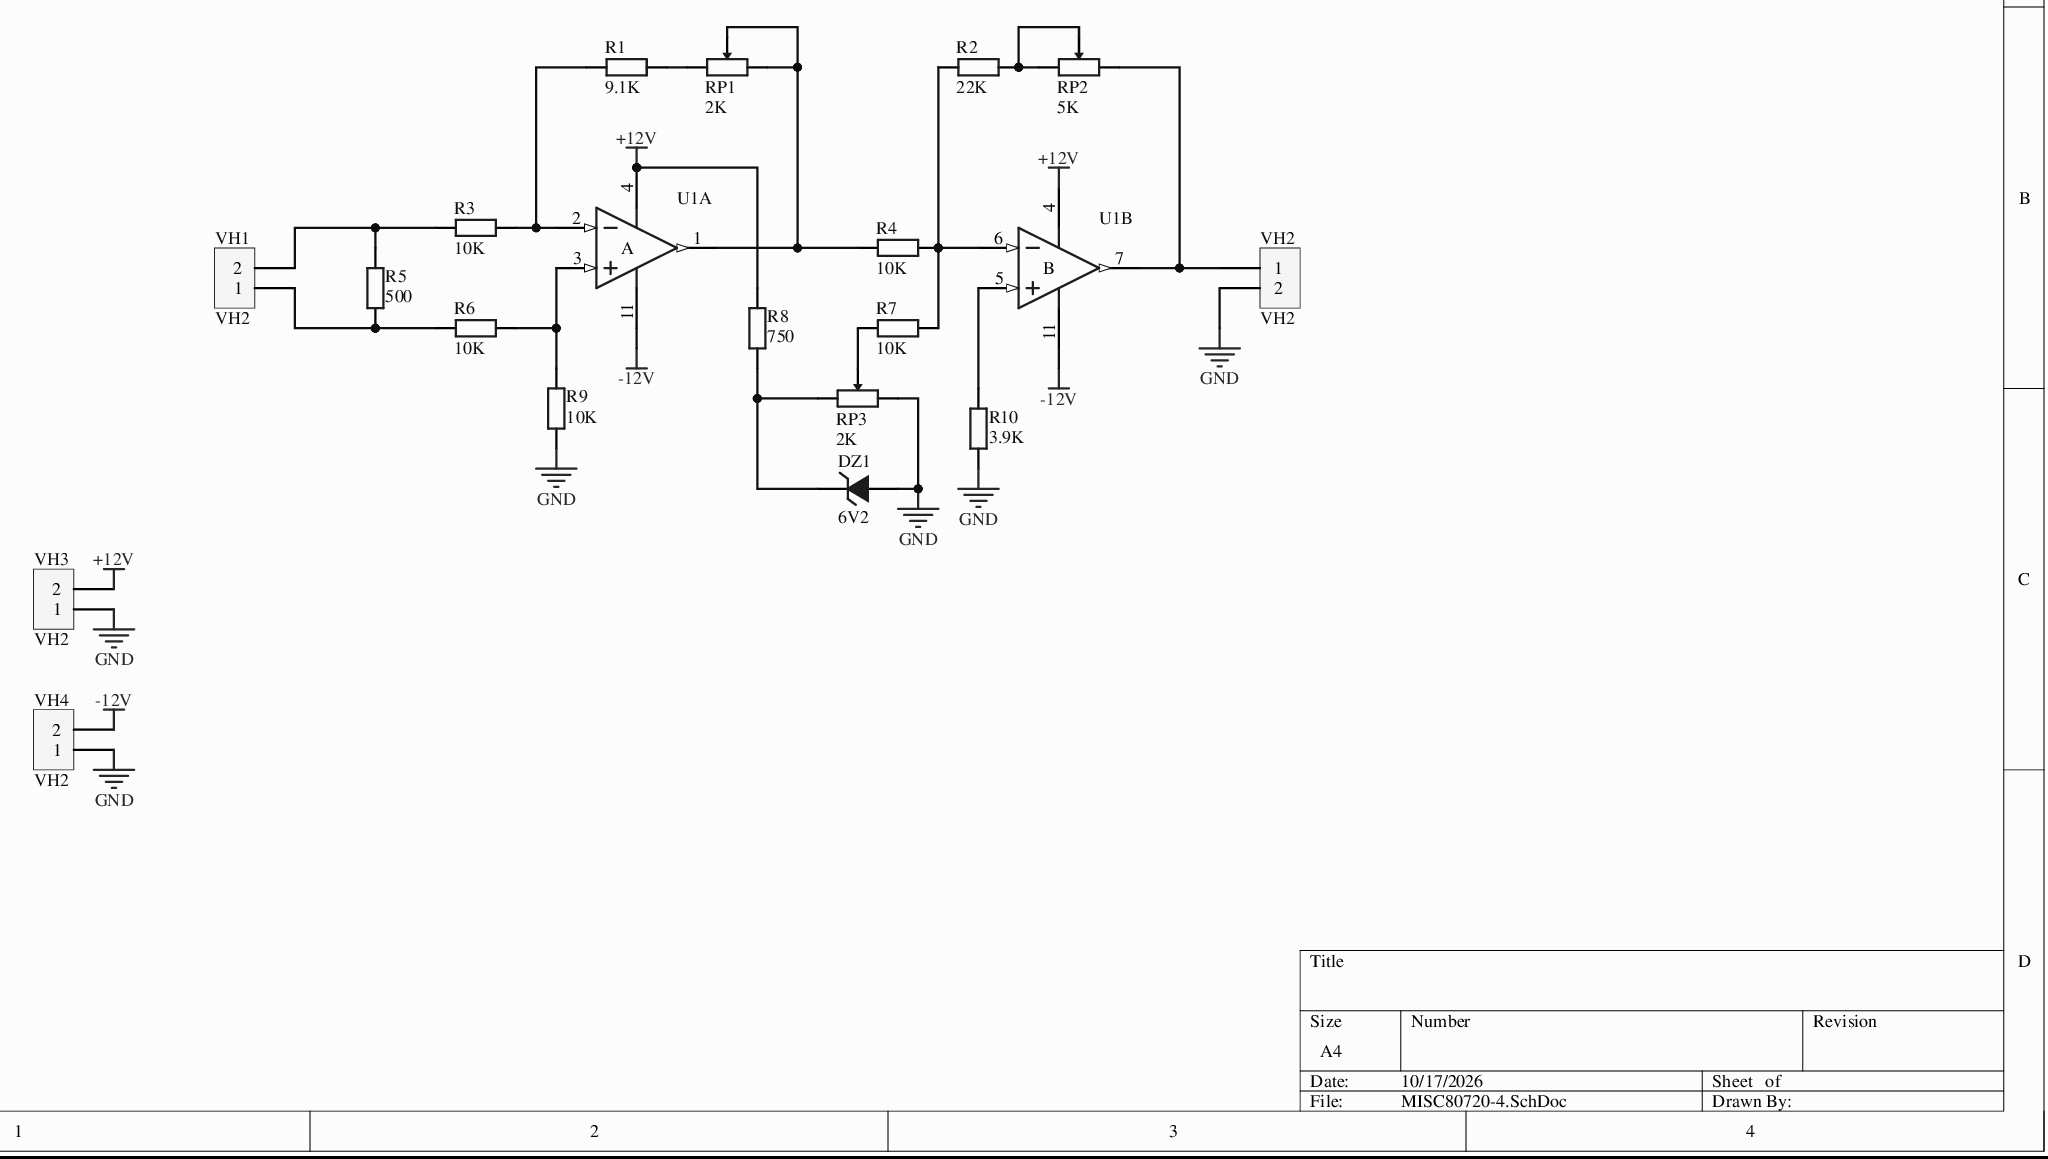
[diagram p0: MISC80720-4.SchDoc]
# Altium project MISC80720-7.PrjPcb
1 sheet, 19 parts. Net scope: global (net labels, ports and power ports of the same name join across sheets).
Board file: MISC80720.PcbDoc

## Sheet MISC80720-4.SchDoc
size A4

### Parts
DZ1  6V2  [DO-35]
R1  9.1K  [RS 1/4W]
R2  22K  [RS 1/4W]
R3  10K  [RS 1/4W]
R4  10K  [RS 1/4W]
R5  500  [RS 1/4W]
R6  10K  [RS 1/4W]
R7  10K  [RS 1/4W]
R8  750  [RS 1/4W]
R9  10K  [RS 1/4W]
R10  3.9K  [RS 1/4W]
RP1  2K  [3296W]
RP2  5K  [3296W]
RP3  2K  [3296W]
U1  LM124AD  [DIP14]  (value not drawn)  (parts A,B of 4)
VH1  VH2  [VH3.96-2A]
VH2  VH2  [VH3.96-2A]
VH3  VH2  [VH3.96-2A]
VH4  VH2  [VH3.96-2A]

### Nets
+12V: R8.2 U1.4(V+) VH3.2
-12V: U1.11(V-) VH4.2
GND: DZ1.1(A) R9.1 R10.1 RP3.3 VH2.2 VH3.1 VH4.1
NetDZ1_2: DZ1.2(K) R8.1 RP3.1
NetR1_1: R1.1 R3.2 U1.2(IN-)
NetR1_2: R1.2 RP1.1
NetR2_1: R2.1 R4.2 R7.2 U1.6(IN-)
NetR2_2: R2.2 RP2.1 RP2.2
NetR3_1: R3.1 R5.2 VH1.2
NetR4_1: R4.1 RP1.2 RP1.3 U1.1(OUT)
NetR5_1: R5.1 R6.1 VH1.1
NetR6_2: R6.2 R9.2 U1.3(IN+)
NetR7_1: R7.1 RP3.2
NetR10_2: R10.2 U1.5(IN+)
NetRP2_3: RP2.3 U1.7(OUT) VH2.1

### Library data of the parts
DZ1 = 1N4106: 12V/0.5W Zener diode; BOM名称: 12V/0.5W Zener diode
R1-R10 = R-S: Color-band resistor; BOM名称: Color-band resistor
RP1-RP3 = RP: Single-gang potentiometer; BOM名称: Through-hole potentiometer
U1 = LM124AD: Low-Power Quad Operational Amplifier; Package Information: Latest Revision: Sep-1998; Published: 24-Aug-2001; Revision: 17-Jul-2002: Re-released for DXP Platform.; Datasheet: Latest Revision: Nov-1997; Package Reference: SO14B; Publisher: Altium Limited